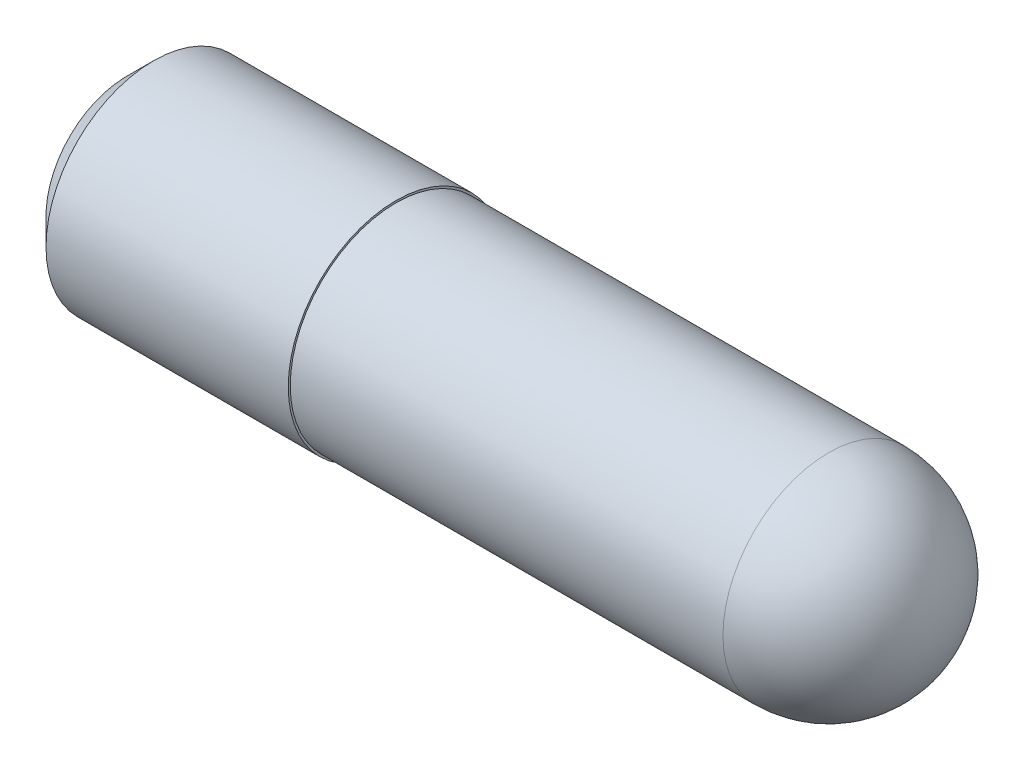
from build123d import *

# Parameters (mm, degrees)
SKETCH_1_R      = 4
EXTRUDE_1_DEPTH = 10
SKETCH_2_R      = 3.925
EXTRUDE_2_DEPTH = 20
FILLET_1_R      = 3.925
CHAMFER_1_SIZE  = 1


with BuildPart() as part:
    # 草图1 → 凸台-拉伸1 (new body)
    with BuildSketch(Plane(origin=(0, 0, 0), x_dir=(0, 0, -1), z_dir=(1, 0, 0))):
        Circle(SKETCH_1_R)
    extrude(amount=EXTRUDE_1_DEPTH)

    # 草图2 → 凸台-拉伸2 (add)
    with BuildSketch(Plane(origin=(10, 0, 0), x_dir=(0, 0, -1), z_dir=(1, 0, 0))):
        Circle(SKETCH_2_R)
    extrude(amount=EXTRUDE_2_DEPTH)

    # 圆角1
    fillet_1_edges = [part.edges().sort_by_distance(p)[0] for p in [
        (30, 0, 3.925),
    ]]
    fillet(fillet_1_edges, radius=FILLET_1_R)

    # 倒角1
    chamfer_1_edges = [part.edges().sort_by_distance(p)[0] for p in [
        (0, 0, 4),
    ]]
    chamfer(chamfer_1_edges, length=CHAMFER_1_SIZE)


solid = part.part
